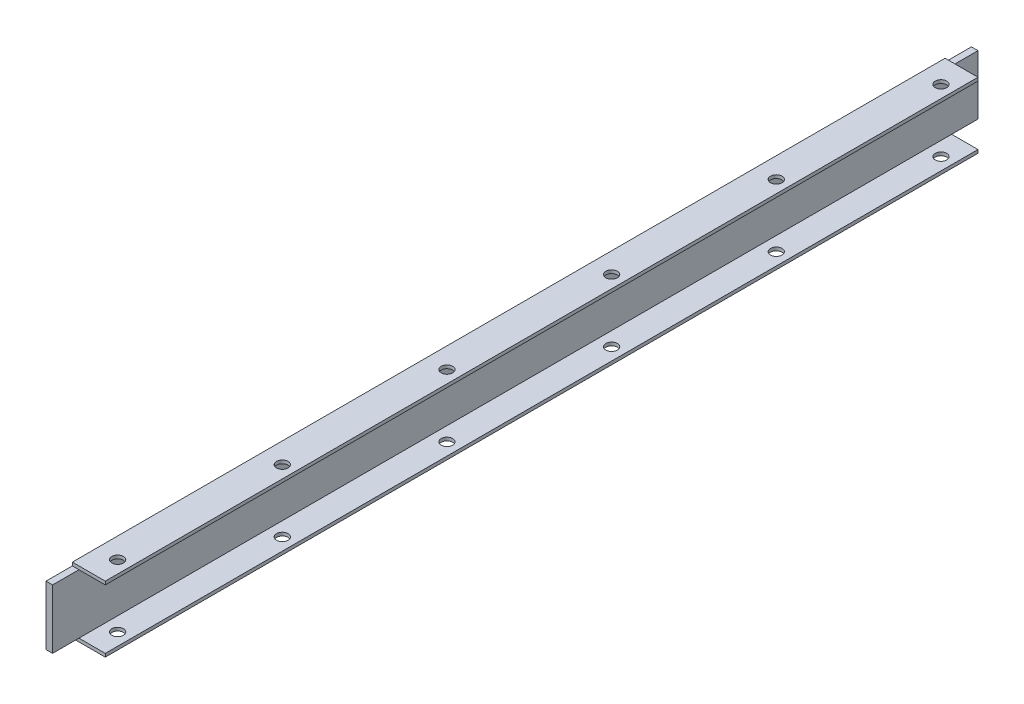
from build123d import *

# Parameters (mm, degrees)
EXTRUDE1_DEPTH     = 1124
SKETCH2_W          = 32
SKETCH2_H          = 32
CUT_EXTRUDE1_DEPTH = 1128.553102962
SKETCH3_W          = 32
SKETCH3_H          = 4
CUT_EXTRUDE2_DEPTH = 1200
SKETCH4_R          = 7
CUT_EXTRUDE3_DEPTH = 1128.553102962
LPATTERN1_COUNT    = 6
LPATTERN1_PITCH    = 200


with BuildPart() as part:
    # Sketch1 → Extrude1 (new body)
    with BuildSketch(Plane.XY):
        Polygon((0, 0), (-40, 0), (-40, 80), (0, 80), (0, 76), (-32, 76), (-32, 4), (0, 4), align=None)
    extrude(amount=EXTRUDE1_DEPTH)

    # Sketch2 → Cut-Extrude1 (cut, through all)
    with BuildSketch(Plane(origin=(0, 80, 0), x_dir=(1, 0, 0), z_dir=(0, 1, 0))):
        with Locations((-16, -16)):
            Rectangle(SKETCH2_W, SKETCH2_H)
        with Locations((-16, -1108)):
            Rectangle(SKETCH2_W, SKETCH2_H)
    extrude(amount=-CUT_EXTRUDE1_DEPTH, mode=Mode.SUBTRACT)

    # Sketch3 → Cut-Extrude2 (cut)
    with BuildSketch(Plane(origin=(-32, 0, 0), x_dir=(0, 0, -1), z_dir=(1, 0, 0))):
        with Locations((-1108, 78)):
            Rectangle(SKETCH3_W, SKETCH3_H)
        with Locations((-1108, 2)):
            Rectangle(SKETCH3_W, SKETCH3_H)
        with Locations((-16, 78)):
            Rectangle(SKETCH3_W, SKETCH3_H)
        with Locations((-16, 2)):
            Rectangle(SKETCH3_W, SKETCH3_H)
    extrude(amount=-CUT_EXTRUDE2_DEPTH, mode=Mode.SUBTRACT)

    # Sketch4 → Cut-Extrude3 (cut, through all)
    with BuildSketch(Plane(origin=(0, 80, 0), x_dir=(1, 0, 0), z_dir=(0, 1, 0))):
        with Locations(Location((-15, -1062, 0), (0, 0, 270))):
            Circle(SKETCH4_R)
    cut_extrude3 = extrude(amount=-CUT_EXTRUDE3_DEPTH, mode=Mode.SUBTRACT)

    # LPattern1: Cut-Extrude3 ×6
    with Locations(*[(0, 0, -i * LPATTERN1_PITCH) for i in range(1, LPATTERN1_COUNT)]):
        add(cut_extrude3, mode=Mode.SUBTRACT)


solid = part.part
